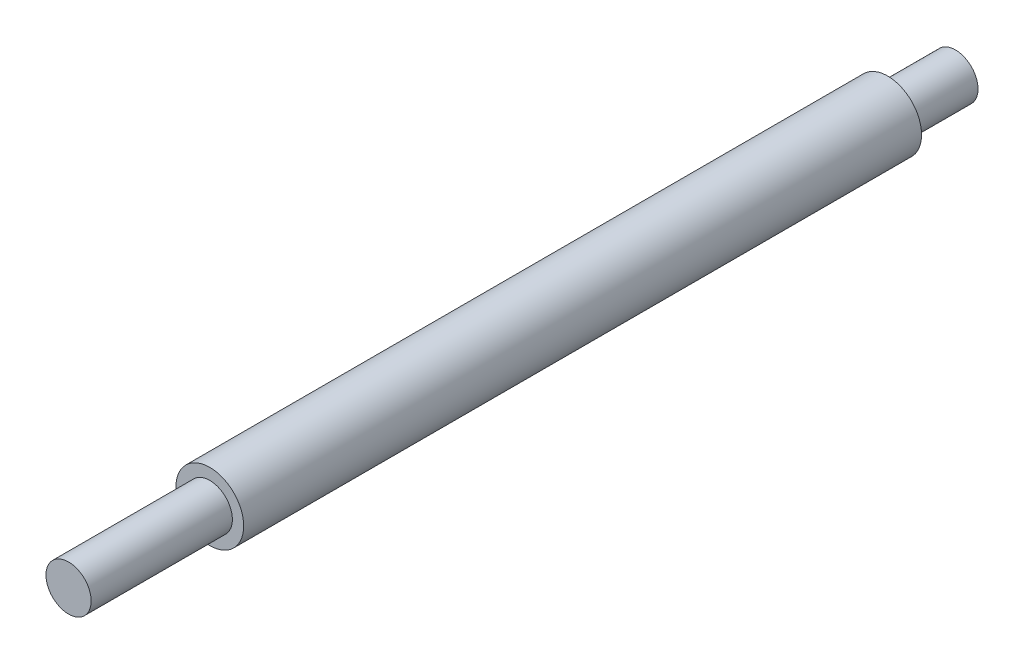
SolidWorks part; units mm, degrees
ref_plane "前视基准面" through (0, 0, 0) normal (0, 0, 1) x (1, 0, 0)
ref_plane "上视基准面" through (0, 0, 0) normal (0, 1, 0) x (1, 0, 0)
ref_plane "右视基准面" through (0, 0, 0) normal (1, 0, 0) x (0, 0, -1)
sketch "草图1" plane through (0, 0, 0) normal (0, 0, 1) x (1, 0, 0)
  circle A0 centre (0, 0) radius 6
  dimension "D1" = 12
extrude "凸台-拉伸1" add sketch "草图1" along normal blind 120
sketch "草图2" plane through (0, 0, 0) normal (0, 0, -1) x (-1, 0, 0)
  circle A0 centre (0, 0) radius 4
  dimension "D1" = 8
extrude "凸台-拉伸2" add sketch "草图2" along normal blind 12
sketch "草图3" plane through (0, 0, 120) normal (0, 0, 1) x (1, 0, 0)
  circle A0 centre (0, 0) radius 4
  dimension "D1" = 8
extrude "凸台-拉伸3" add sketch "草图3" along normal blind 25
